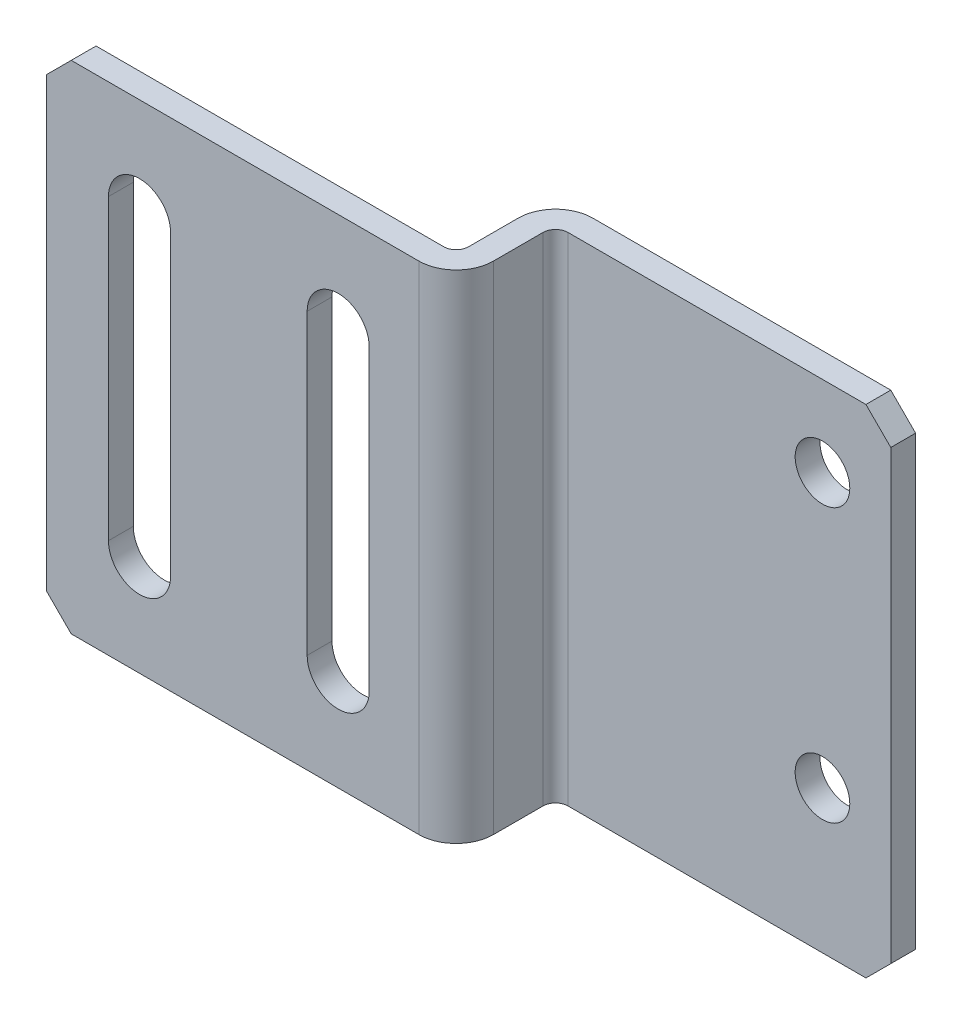
SolidWorks part; units mm, degrees
ref_plane "Front Plane" through (0, 0, 0) normal (0, 0, 1) x (1, 0, 0)
ref_plane "Top Plane" through (0, 0, 0) normal (0, 1, 0) x (1, 0, 0)
ref_plane "Right Plane" through (0, 0, 0) normal (1, 0, 0) x (0, 0, -1)
sketch "Sketch1" plane through (0, 0, 0) normal (0, 1, 0) x (1, 0, 0)
  line L1 (0, 0) -> (16.5, 0)
  line L2 (0, 0) -> (0, 1)
  line L3 (15.5, 5) -> (30, 5)
  line L4 (30, 4) -> (30, 5)
  line L7 (0, 1) -> (15.5, 1)
  line L8 (15.5, 5) -> (15.5, 1)
  line L11 (30, 4) -> (16.5, 4)
  line L12 (16.5, 0) -> (16.5, 4)
  dimension "D1" = 1
  dimension "D2" = 1
  dimension "D3" = 1
  dimension "D4" = 14.5
  dimension "D5" = 30
  dimension "D6" = 5
extrude "Boss-Extrude1" add sketch "Sketch1" along normal blind 20
sketch "Sketch2" plane through (0, 0, -5) normal (0, 0, -1) x (-1, 0, 0)
  line L0 (-7.75, 20) -> (-7.75, -49980) construction
  line L1 (-15.5, 20) -> (0, 20) construction
  line L2 (0, 10) -> (-50000, 10) construction
  line L3 (0, 20) -> (0, 0) construction
  line L4 (-11.75, 16) -> (-11.75, 4) construction
  line L5 (-10.5, 16) -> (-10.5, 4)
  line L6 (-13, 16) -> (-13, 4)
  line L7 (-11, 10) -> (49989, 10) construction
  line L8 (-3.75, 16) -> (-3.75, 4) construction
  line L9 (-5, 16) -> (-5, 4)
  line L10 (-2.5, 16) -> (-2.5, 4)
  arc A0 (-10.5, 16) -> (-13, 16) centre (-11.75, 16) ccw
  arc A1 (-13, 4) -> (-10.5, 4) centre (-11.75, 4) ccw
  arc A2 (-5, 16) -> (-2.5, 16) centre (-3.75, 16) cw
  arc A3 (-2.5, 4) -> (-5, 4) centre (-3.75, 4) cw
  point P4 (-7.75, 20)
  point P9 (0, 10)
  point P12 (-11.75, 10)
  point P21 (-3.75, 10)
  dimension "D1" = 2.5
  dimension "D2" = 8
  dimension "D3" = 12
extrude "Cut-Extrude1" cut sketch "Sketch2" against normal blind 10
chamfer "Chamfer1" distance 1 angle 45 4 edges at (30, 0, -4.5) (30, 20, -4.5) (0, 0, -0.5) (0, 20, -0.5)
fillet "Fillet1" radius 1.5 2 edges at (15.5, 10, -5) (16.5, 10, 0)
fillet "Fillet2" radius 0.5 2 edges at (16.5, 10, -4) (15.5, 10, -1)
hole_wizard "Ø2.2 (2.2) Diameter Hole1" positions "Sketch4" profile "Sketch3" hole size "Ø2.2" standard "Gb"
sketch "Sketch4" plane through (0, 0, -4) normal (0, 0, 1) x (1, 0, 0)
  line L0 (30, 19) -> (30, 1) construction
  line L1 (17, 20) -> (29, 20) construction
  point P0 (27.25, 16.75)
  point P3 (27.25, 5.75)
  dimension "D1" = 2.75
  dimension "D2" = 3.25
  dimension "D3" = 11
sketch "Sketch3" plane through (27.25, 16.75, -4) normal (1, 0, 0) x (0, -1, 0)
  line L0 (0, 0) -> (0, 5.6609)
  line L1 (0, 5.6609) -> (1.1, 5)
  line L2 (1.1, 5) -> (1.1, 0)
  line L5 (1.1, 0) -> (0, 0)
  line L10 (0, 5.6609) -> (-1.1, 5) construction
  line L11 (0, -6.35) -> (0, 107.95) construction
  dimension "孔直径" = 2.2
  dimension "孔深度" = 5
  dimension "导头角度" = 118
